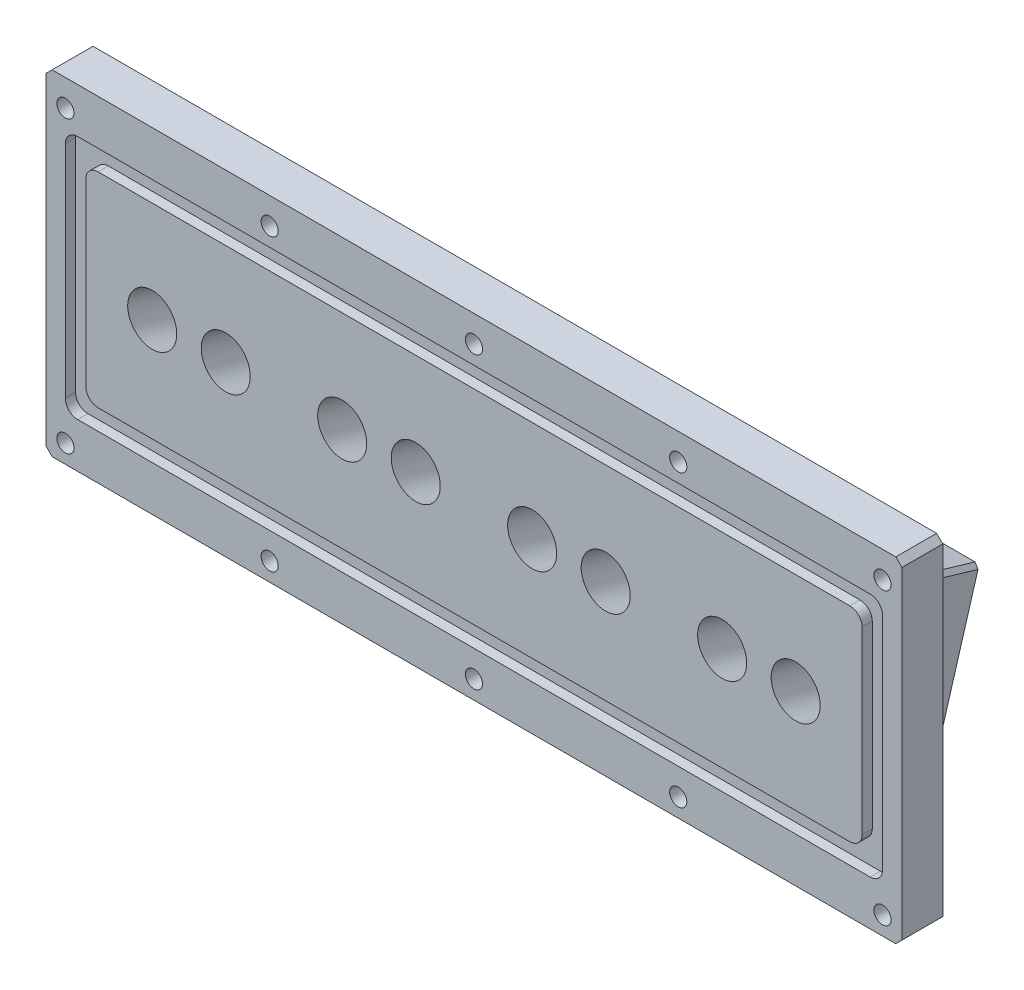
from build123d import *

# Parameters (mm, degrees)
SKETCH1_W             = 419
SKETCH1_H             = 164
BOSS_EXTRUDE1_DEPTH   = 20
SKETCH2_W             = 400
SKETCH2_H             = 120
SKETCH2_W_2           = 380
SKETCH2_H_2           = 100
CUT_EXTRUDE1_DEPTH    = 5
FILLET1_R             = 6
CHAMFER1_SIZE         = 3
HOLE1_D               = 8.4
HOLE1_CBORE_D         = 15
HOLE1_CBORE_DEPTH     = 11
BOSS_EXTRUDE2_DEPTH   = 379
CHAMFER2_SIZE         = 2
HOLE2_D               = 24
M6_TAPPED_HOLE1_D     = 5
M6_TAPPED_HOLE1_DEPTH = 12
M6_TAPPED_HOLE1_TIP   = 1.502151548
SKETCH12_W            = 359
SKETCH12_H            = 78
CUT_EXTRUDE2_DEPTH    = 15
FILLET2_R             = 6


with BuildPart() as part:
    # Sketch1 → Boss-Extrude1 (new body)
    with BuildSketch(Plane.XY):
        Rectangle(SKETCH1_W, SKETCH1_H)
    extrude(amount=BOSS_EXTRUDE1_DEPTH)

    # Sketch2 → Cut-Extrude1 (cut)
    with BuildSketch(Plane.XY.offset(20)):
        Rectangle(SKETCH2_W, SKETCH2_H)
        Rectangle(SKETCH2_W_2, SKETCH2_H_2, mode=Mode.SUBTRACT)
    extrude(amount=-CUT_EXTRUDE1_DEPTH, mode=Mode.SUBTRACT)

    # Fillet1
    fillet1_edges = [part.edges().sort_by_distance(p)[0] for p in [
        (200, 60, 17.5),
        (200, -60, 17.5),
        (-200, -60, 17.5),
        (-200, 60, 17.5),
        (190, -50, 17.5),
        (-190, -50, 17.5),
        (-190, 50, 17.5),
        (190, 50, 17.5),
    ]]
    fillet(fillet1_edges, radius=FILLET1_R)

    # Chamfer1
    chamfer1_edges = [part.edges().sort_by_distance(p)[0] for p in [
        (209.5, -82, 10),
        (-209.5, -82, 10),
        (-209.5, 82, 10),
        (209.5, 82, 10),
    ]]
    chamfer(chamfer1_edges, length=CHAMFER1_SIZE)

    # Hole1 (through all)
    with Locations(Plane(origin=(0, 0, 0), x_dir=(-1, 0, 0), z_dir=(0, 0, -1))):
        with Locations((-200, 69), (-200, -73), (-100, -73), (0, -73), (100, -73), (200, -73), (200, 69), (100, 69), (0, 69), (-100, 69)):
            CounterBoreHole(HOLE1_D / 2, HOLE1_CBORE_D / 2, HOLE1_CBORE_DEPTH)

    # Sketch6 → Boss-Extrude2 (add)
    with BuildSketch(Plane.ZY.offset(189.5)):
        Polygon((0, 52.67), (-37.82, 41.470170836), (-6.578312083, -64), (0, -64), align=None)
    extrude(amount=-BOSS_EXTRUDE2_DEPTH)

    # Chamfer2
    chamfer2_edges = [part.edges().sort_by_distance(p)[0] for p in [
        (189.5, -64, -3.289156041),
        (189.5, 47.070085418, -18.91),
        (-189.5, 47.070085418, -18.91),
        (-189.5, -64, -3.289156041),
    ]]
    chamfer(chamfer2_edges, length=CHAMFER2_SIZE)

    # Hole2 (through all)
    with Locations(Plane(origin=(0, -6.953944598, -23.476123527), x_dir=(-1, 0, 0), z_dir=(0, -0.2840153447039166, -0.9588197348681949))):
        with Locations((157.5, -5.198964564), (121.5, -5.198964564), (64.5, -5.198964564), (28.5, -5.198964564), (-28.5, -5.198964564), (-64.5, -5.198964564), (-121.5, -5.198964564), (-157.5, -5.198964564)):
            Hole(HOLE2_D / 2)

    # M6 Tapped Hole1
    with Locations(Plane(origin=(0, -6.953944598, -23.476123527), x_dir=(-1, 0, 0), z_dir=(0, -0.2840153447039166, -0.9588197348681949))):
        with Locations((-169.5, 39.801035436), (-109.5, 39.801035436), (-76.5, 39.801035436), (-16.5, 39.801035436), (16.5, 39.801035436), (76.5, 39.801035436), (109.5, 39.801035436), (169.5, 39.801035436), (169.5, -50.198964564), (109.5, -50.198964564), (76.5, -50.198964564), (16.5, -50.198964564), (-16.5, -50.198964564), (-76.5, -50.198964564), (-109.5, -50.198964564), (-169.5, -50.198964564)):
            Hole(M6_TAPPED_HOLE1_D / 2, depth=M6_TAPPED_HOLE1_DEPTH)
            with Locations((0, 0, -(M6_TAPPED_HOLE1_DEPTH + M6_TAPPED_HOLE1_TIP / 2))):  # 118° drill point
                Cone(0, M6_TAPPED_HOLE1_D / 2, M6_TAPPED_HOLE1_TIP, mode=Mode.SUBTRACT)

    # Sketch12 → Cut-Extrude2 (cut)
    with BuildSketch(Plane(origin=(0, -6.953944598, -23.476123527), x_dir=(-1, 0, 0), z_dir=(0, -0.2840153447039166, -0.9588197348681949))):
        with Locations((0, -5.196121458)):
            Rectangle(SKETCH12_W, SKETCH12_H)
    extrude(amount=-CUT_EXTRUDE2_DEPTH, mode=Mode.SUBTRACT)

    # Fillet2
    fillet2_edges = [part.edges().sort_by_distance(p)[0] for p in [
        (179.5, -47.199942971, -3.732598845),
        (179.5, 27.587996348, -25.885795732),
        (-179.5, 27.587996348, -25.885795732),
        (-179.5, -47.199942971, -3.732598845),
    ]]
    fillet(fillet2_edges, radius=FILLET2_R)


solid = part.part
